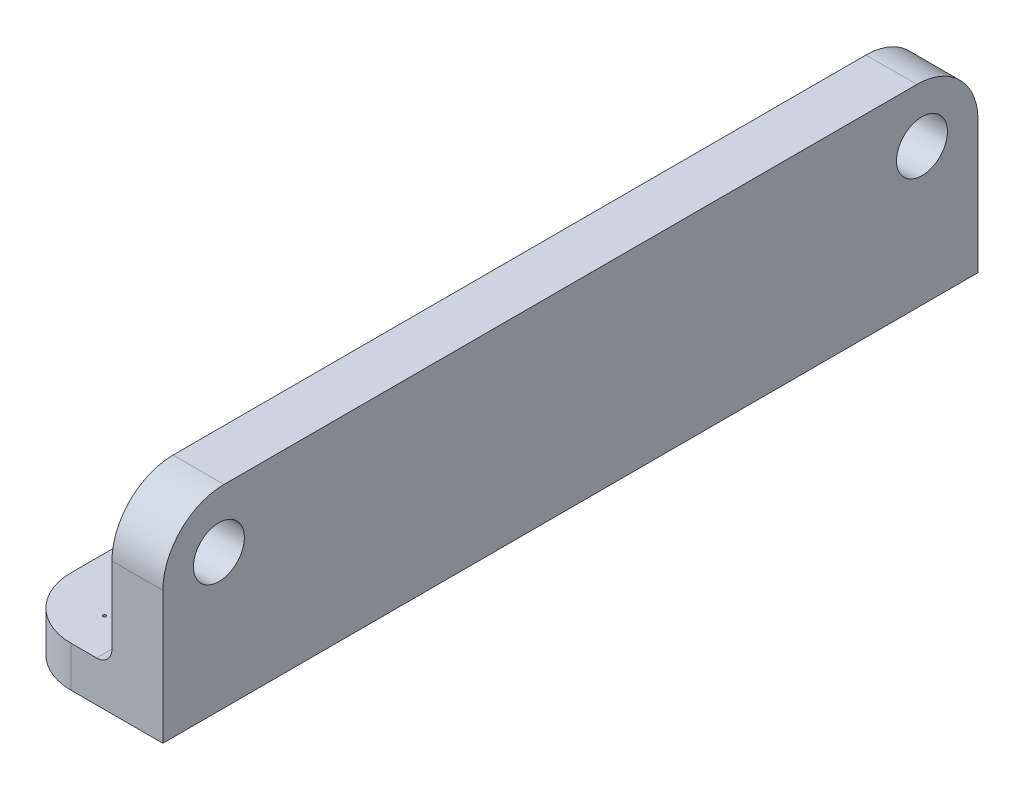
SolidWorks part; units mm, degrees
ref_plane "Front Plane" through (0, 0, 0) normal (0, 0, 1) x (1, 0, 0)
ref_plane "Top Plane" through (0, 0, 0) normal (0, 1, 0) x (1, 0, 0)
ref_plane "Right Plane" through (0, 0, 0) normal (1, 0, 0) x (0, 0, -1)
sketch "Sketch1" plane through (0, 0, 0) normal (0, 0, 1) x (1, 0, 0)
  line L0 (0, 0) -> (0, 38)
  line L1 (0, 38) -> (-10, 38)
  line L2 (-10, 38) -> (-10, 11)
  line L3 (-13, 8) -> (-30, 8)
  line L4 (-30, 8) -> (-30, 0)
  line L5 (-30, 0) -> (0, 0)
  arc A0 (-10, 11) -> (-13, 8) centre (-13, 11) cw
  point P9 (-10, 8)
  dimension "D5" = 3
  dimension "D1" = 30
  dimension "D2" = 8
  dimension "D3" = 10
  dimension "D4" = 30
extrude "Boss-Extrude1" add sketch "Sketch1" along normal blind 160
sketch "Sketch2" plane through (0, 0, 0) normal (1, 0, 0) x (0, 0, -1)
  line L0 (0, 0) -> (0, 38) construction
  line L1 (-160, 38) -> (0, 38) construction
  circle A0 centre (-149, 27) radius 5
  circle A1 centre (-11, 27) radius 5
  point P4 (0, 0)
  dimension "D3" = 10
  dimension "D1" = 11
  dimension "D2" = 138
  dimension "D4" = 11
extrude "Cut-Extrude1" cut sketch "Sketch2" against normal blind 10
fillet "Fillet1" radius 12 2 edges at (-5, 38, 0) (-5, 38, 160)
sketch "Sketch3" plane through (0, 0, 0) normal (0, -1, 0) x (1, 0, 0)
  line L0 (-30, 160) -> (0, 160) construction
  line L1 (0, 160) -> (0, 0) construction
  circle A0 centre (-19.4, 152.04) radius 0.29
  circle A1 centre (-19.4, 132.04) radius 0.29
  circle A2 centre (-19.4, 112.04) radius 0.29
  circle A3 centre (-19.4, 92.04) radius 0.29
  circle A4 centre (-19.4, 72.04) radius 0.29
  circle A5 centre (-19.4, 52.04) radius 0.29
  circle A6 centre (-19.4, 32.04) radius 0.29
  circle A7 centre (-19.4, 12.04) radius 0.29
  point P16 (0, 0)
  point P21 (-20.8776, 153.1201)
  dimension "D1" = 0.58
  dimension "D2" = 7.96
  dimension "D3" = 19.4
  dimension "D4" = 20
  dimension "D5" = 20
  dimension "D6" = 20
  dimension "D7" = 20
  dimension "D8" = 20
  dimension "D9" = 20
  dimension "D10" = 20
extrude "Cut-Extrude2" cut sketch "Sketch3" against normal blind 10
fillet "Fillet2" radius 12 2 edges at (-30, 4, 0) (-30, 4, 160)
sketch "Sketch4" plane through (-10, 0, 0) normal (-1, 0, 0) x (0, 0, 1)
  line L0 (11, 22) -> (149, 22) construction
  circle A0 centre (11, 27) radius 5 construction
  circle A1 centre (149, 27) radius 5 construction
  text T0 "               OLD  AMALGAMATED" font "Century Gothic" height 5
  point P6 (0, 0)
  point P7 (0, 0)
  dimension "D1" = 138
extrude "Cut-Extrude3" cut sketch "Sketch4" against normal blind 2
